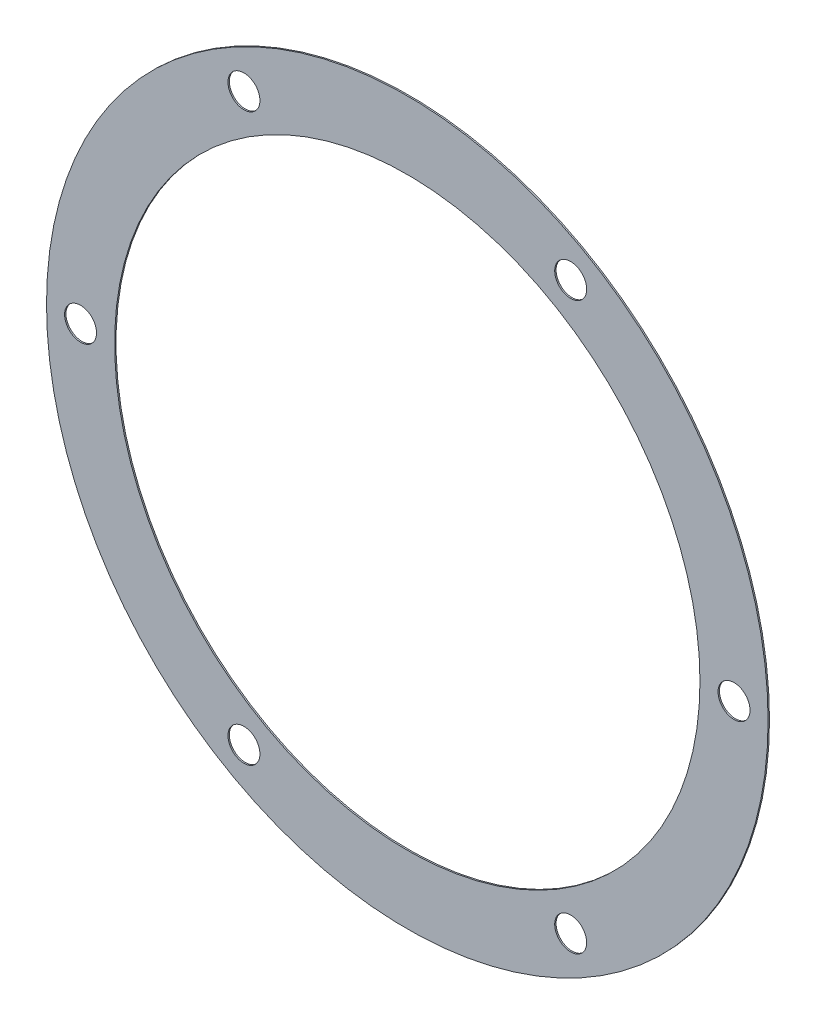
SolidWorks part; units mm, degrees
material "NY250"
ref_plane "Front Plane" through (0, 0, 0) normal (0, 0, 1) x (1, 0, 0)
ref_plane "Top Plane" through (0, 0, 0) normal (0, 1, 0) x (1, 0, 0)
ref_plane "Right Plane" through (0, 0, 0) normal (1, 0, 0) x (0, 0, -1)
sketch "Sketch1" plane through (0, 0, 0) normal (0, 0, 1) x (1, 0, 0)
  circle A0 centre (0, 0) radius 259.5
  circle A1 centre (0, 0) radius 210.5
  dimension "D1" = 519
  dimension "D2" = 421
extrude "Boss-Extrude1" add sketch "Sketch1" along normal blind 1
sketch "Sketch2" plane through (0, 0, 1) normal (0, 0, 1) x (1, 0, 0)
  circle A0 centre (-235, 0) radius 11.5
  dimension "D1" = 23
  dimension "D2" = 235
  dimension "D3" = 0
extrude "Cut-Extrude1" cut sketch "Sketch2" against normal up to next
pattern_circular "CirPattern1" count 6 over 360 about axis through (0, 0, 0) along (0, 0, 1) of "Cut-Extrude1"
